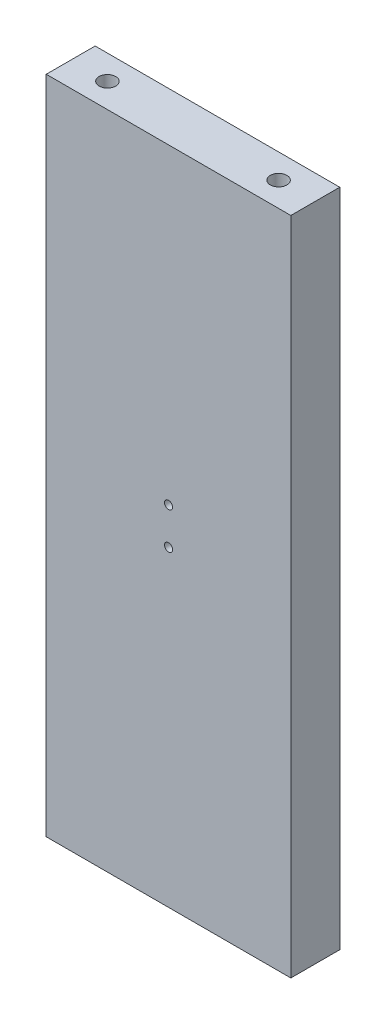
SolidWorks part; units mm, degrees
material "普通碳钢"
ref_plane "Front Plane" through (0, 0, 0) normal (0, 0, 1) x (1, 0, 0)
ref_plane "Top Plane" through (0, 0, 0) normal (0, 1, 0) x (1, 0, 0)
ref_plane "Right Plane" through (0, 0, 0) normal (1, 0, 0) x (0, 0, -1)
sketch "Sketch1" plane through (0, 0, 0) normal (0, 0, 1) x (1, 0, 0)
  line L1 (0, 0) -> (100, 0)
  line L2 (0, 0) -> (0, -270)
  line L3 (0, -270) -> (100, -270)
  line L4 (100, 0) -> (100, -270)
  line L5 (0, 0) -> (100, -270) construction
  line L6 (0, -270) -> (100, 0) construction
  point P4 (50, -135)
  dimension "D1" = 270
  dimension "D2" = 100
extrude "Boss-Extrude1" add sketch "Sketch1" along normal blind 20
hole_wizard "M8 Tapped Hole1" positions "3DSketch1" profile "Sketch2" tap size "M8" standard "GB"
sketch3d "3DSketch1"
  line L0 (0, 0, 10) -> (100, 0, 10) construction
  line L1 (0, 0, 20) -> (0, 0, 0) construction
  line L2 (100, 0, 20) -> (100, 0, 0) construction
  line L3 (0, -270, 10) -> (100, -270, 10) construction
  line L4 (0, -270, 20) -> (0, -270, 0) construction
  line L5 (100, -270, 20) -> (100, -270, 0) construction
  point P0 (15, 0, 10)
  point P2 (85, 0, 10)
  point P12 (15, -270, 10)
  point P14 (85, -270, 10)
  dimension "D1" = 70
  dimension "D2" = 15
  dimension "D3" = 70
  dimension "D4" = 15
sketch "Sketch2" plane through (15, 0, 10) normal (1, 0, 0) x (0, 0, 1)
  line L0 (0, 0) -> (0, 21.7929)
  line L1 (0, 21.7929) -> (3.4, 19.75)
  line L2 (3.4, 19.75) -> (3.4, 0)
  line L5 (3.4, 0) -> (0, 0)
  line L10 (0, 21.7929) -> (-3.4, 19.75) construction
  line L11 (0, -6.35) -> (0, 107.95) construction
  dimension "螺纹孔钻头直径" = 6.8
  dimension "螺纹孔钻头深度" = 19.75
  dimension "导头角度" = 118
cosmetic thread "Hole Cosmetic Thread1"
cosmetic thread "Hole Cosmetic Thread2"
cosmetic thread "Hole Cosmetic Thread3"
cosmetic thread "Hole Cosmetic Thread4"
hole_wizard "M4 Tapped Hole2" positions "Sketch3" profile "Sketch4" tap size "M4" standard "GB"
sketch "Sketch3" plane through (0, 0, 20) normal (0, 0, 1) x (1, 0, 0)
  line L0 (0, -135) -> (12.5134, -135) construction
  line L1 (0, 0) -> (0, -270) construction
  line L3 (50, -142.5) -> (50, -270) construction
  line L4 (0, -270) -> (100, -270) construction
  point P0 (50, -127.5)
  point P2 (50, -142.5)
  dimension "D1" = 15
sketch "Sketch4" plane through (50, -127.5, 20) normal (1, 0, 0) x (0, -1, 0)
  line L0 (0, 0) -> (0, 11.0914)
  line L1 (0, 11.0914) -> (1.65, 10.1)
  line L2 (1.65, 10.1) -> (1.65, 0)
  line L5 (1.65, 0) -> (0, 0)
  line L10 (0, 11.0914) -> (-1.65, 10.1) construction
  line L11 (0, -6.35) -> (0, 107.95) construction
  dimension "螺纹孔钻头直径" = 3.3
  dimension "螺纹孔钻头深度" = 10.1
  dimension "导头角度" = 118
cosmetic thread "Hole Cosmetic Thread5" parameters "D1"=8, "D2"=4
cosmetic thread "Hole Cosmetic Thread6" parameters "D1"=8, "D2"=4
hole_wizard "M4 Tapped Hole1" positions "Sketch6" profile "Sketch7" tap size "M4" standard "GB"
sketch "Sketch6" plane through (0, 0, 0) normal (0, 0, -1) x (-1, 0, 0)
  line L0 (-100, -270) -> (-100, 0) construction
  line L1 (-100, 0) -> (0, 0) construction
  point P0 (-60, -55)
  point P2 (-60, -115)
  point P4 (-60, -175)
  dimension "D1" = 40
  dimension "D2" = 55
  dimension "D3" = 60
  dimension "D4" = 60
sketch "Sketch7" plane through (60, -55, 0) normal (1, 0, 0) x (0, 1, 0)
  line L0 (0, 0) -> (0, 11.0914)
  line L1 (0, 11.0914) -> (1.65, 10.1)
  line L2 (1.65, 10.1) -> (1.65, 0)
  line L5 (1.65, 0) -> (0, 0)
  line L10 (0, 11.0914) -> (-1.65, 10.1) construction
  line L11 (0, -6.35) -> (0, 107.95) construction
  dimension "螺纹孔钻头直径" = 3.3
  dimension "螺纹孔钻头深度" = 10.1
  dimension "导头角度" = 118
cosmetic thread "Hole Cosmetic Thread7"
cosmetic thread "Hole Cosmetic Thread8"
cosmetic thread "Hole Cosmetic Thread9"
